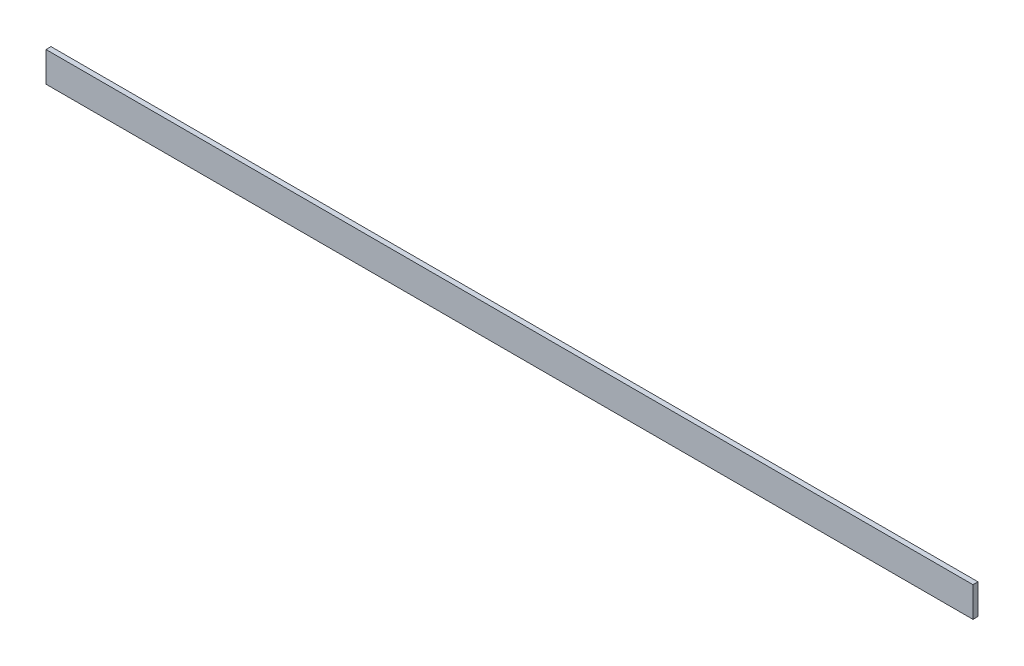
SolidWorks part; units mm, degrees
material "1023 碳钢板 (SS)"
ref_plane "Front Plane" through (0, 0, 0) normal (0, 0, 1) x (1, 0, 0)
ref_plane "Top Plane" through (0, 0, 0) normal (0, 1, 0) x (1, 0, 0)
ref_plane "Right Plane" through (0, 0, 0) normal (1, 0, 0) x (0, 0, -1)
sketch "Sketch1" plane through (0, 0, 0) normal (0, 0, 1) x (1, 0, 0)
  line L1 (-462.5, 15) -> (462.5, 15)
  line L2 (-462.5, 15) -> (-462.5, -15)
  line L3 (-462.5, -15) -> (462.5, -15)
  line L4 (462.5, 15) -> (462.5, -15)
  line L5 (-462.5, 15) -> (462.5, -15) construction
  line L6 (-462.5, -15) -> (462.5, 15) construction
  point P0 (0, 0)
  dimension "D1" = 925
  dimension "D2" = 30
extrude "Boss-Extrude1" add sketch "Sketch1" along normal blind 5
